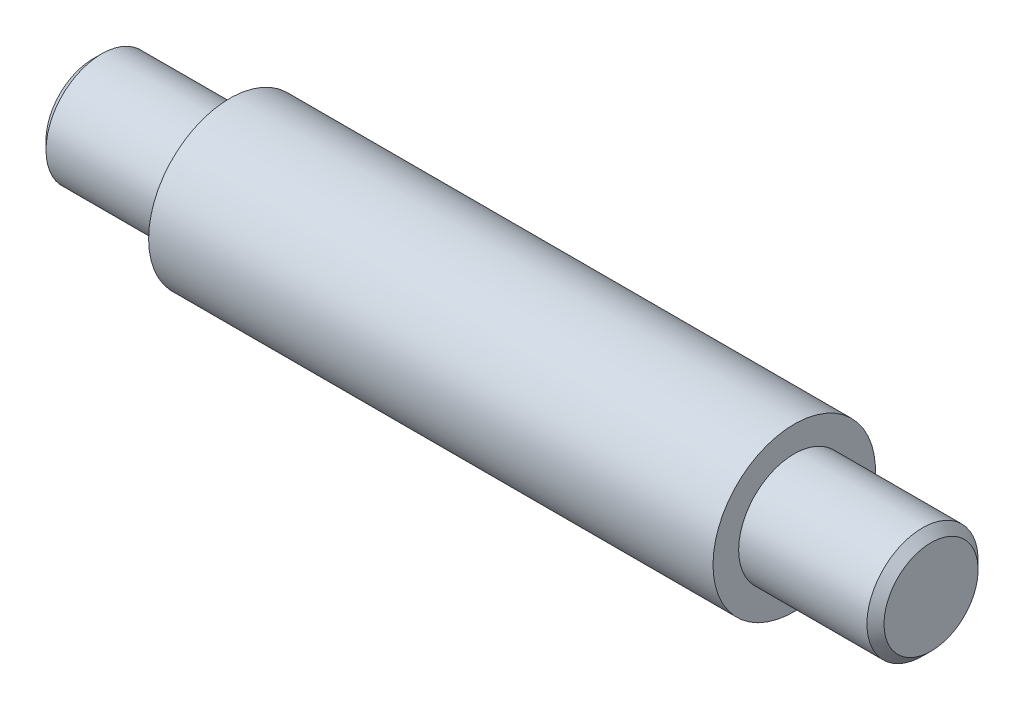
from build123d import *

# Parameters (mm, degrees)
CHAMFER1_SIZE = 25.4


with BuildPart() as part:
    # Sketch1 → Revolve1 (revolve)
    with BuildSketch(Plane.XY, mode=Mode.PRIVATE) as revolve1_sk:
        Polygon((-1244.6, 0), (1244.6, 0), (1244.6, 165.1), (838.2, 165.1), (838.2, 241.3), (-838.2, 241.3), (-838.2, 165.1), (-1244.6, 165.1), align=None)
    revolve(revolve1_sk.sketch.rotate(Axis((-1244.6, 0, 0), (1, 0, 0)), 90), axis=Axis((-1244.6, 0, 0), (1, 0, 0)))

    # Chamfer1
    chamfer1_edges = [part.edges().sort_by_distance(p)[0] for p in [
        (-1244.6, 0, -165.1),
        (1244.6, 0, -165.1),
    ]]
    chamfer(chamfer1_edges, length=CHAMFER1_SIZE)


solid = part.part
